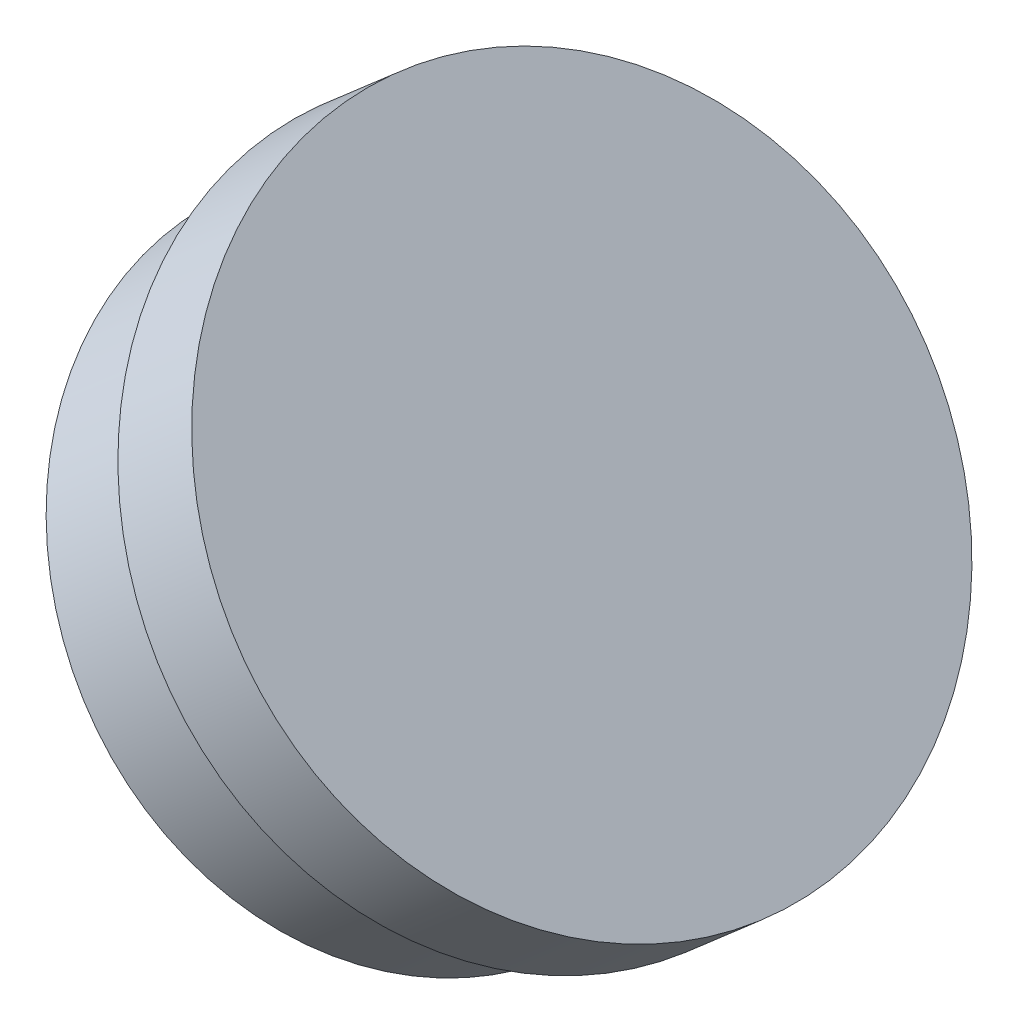
from build123d import *

# Parameters (mm, degrees)
CHAMFER1_SIZE = 0.5


with BuildPart() as part:
    # Sketch1 → Revolve1 (revolve)
    with BuildSketch(Plane.XY):
        Polygon((1431.493261903, -44.982204273), (1430.837202874, -44.227494693), (1433.101331614, -42.259317606), (1439.661921904, -49.806413409), (1433.624245262, -55.05488564), (1427.719714002, -48.262499418), align=None)
    revolve(axis=Axis((1439.661921904, -49.806413409, 0), (-0.7547095802227773, -0.6560590289905012, 0)))

    # Chamfer1
    chamfer1_edges = [part.edges().sort_by_distance(p)[0] for p in [
        (1439.528776523, -61.847271862, 0),
    ]]
    chamfer(chamfer1_edges, length=CHAMFER1_SIZE)


solid = part.part
